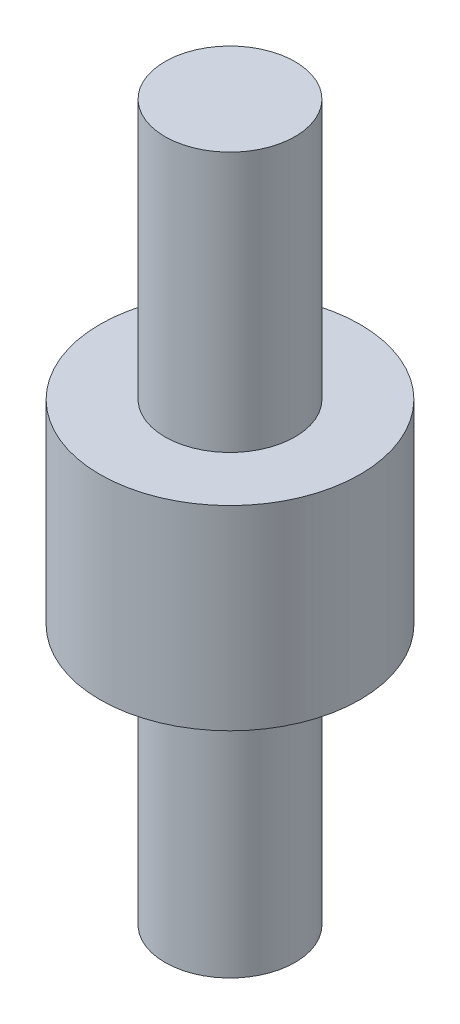
from build123d import *

# Parameters (mm, degrees)
CUT_EXTRUDE1_DEPTH = 2.5


with BuildPart() as part:
    # Sketch1 → Revolve1 (revolve)
    with BuildSketch(Plane(origin=(0, 0, 0), x_dir=(0, 0, -1), z_dir=(1, 0, 0))):
        Polygon((0, 55), (-10, 55), (-10, 15), (-20, 15), (-20, -15), (-10, -15), (-10, -55), (0, -55), align=None)
    revolve(axis=Axis((0, 189.929754582, 0), (0, -1, 0)))

    # Sketch2 → Cut-Extrude1 (cut)
    with BuildSketch(Plane(origin=(0, 0, -10), x_dir=(-1, 0, 0), z_dir=(0, 0, -1))):
        with BuildLine():
            Line((2.5, 45), (2.5, 25))
            ThreePointArc((2.5, 25), (0, 22.5), (-2.5, 25))
            Line((-2.5, 25), (-2.5, 45))
            ThreePointArc((-2.5, 45), (0, 47.5), (2.5, 45))
        make_face()
    cut_extrude1 = extrude(amount=-CUT_EXTRUDE1_DEPTH, mode=Mode.SUBTRACT)

    # Mirror1: Cut-Extrude1 across plane
    add(cut_extrude1.mirror(Plane.ZX), mode=Mode.SUBTRACT)


solid = part.part
